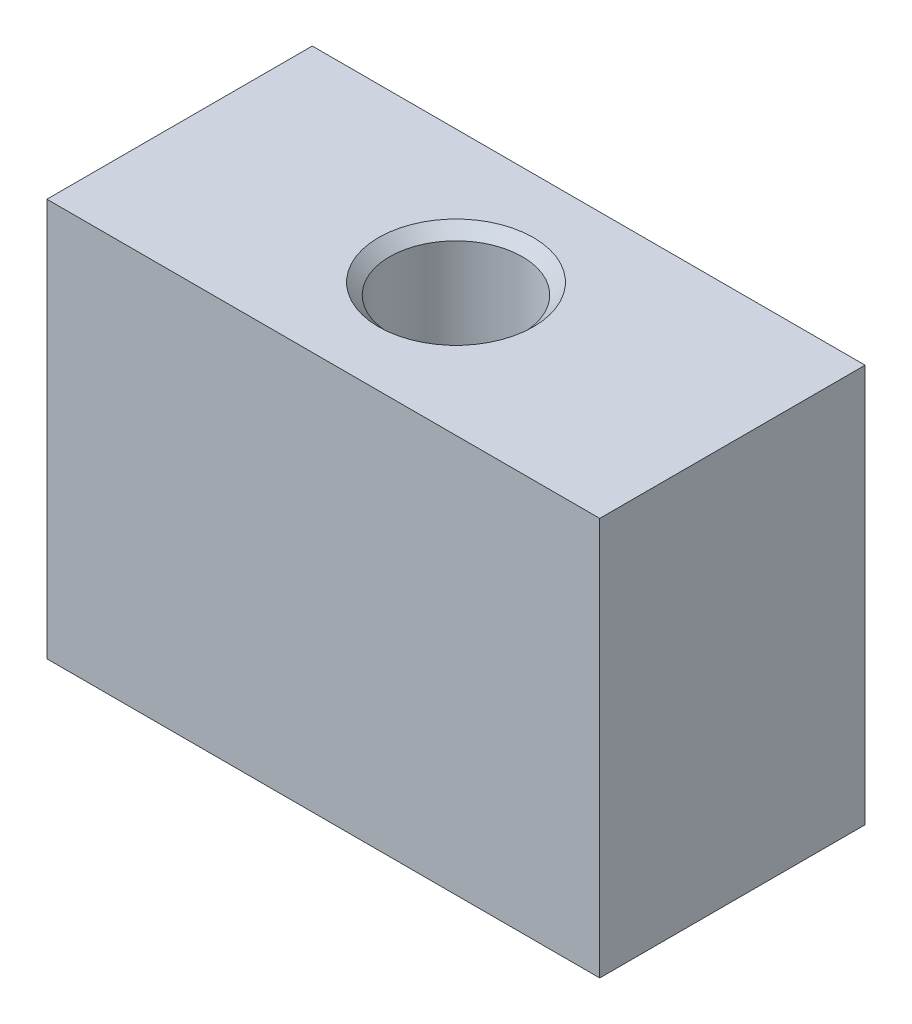
from build123d import *

# Parameters (mm, degrees)
SKETCH1_W           = 25
SKETCH1_H           = 12
BOSS_EXTRUDE1_DEPTH = 18
SKETCH2_R           = 3
CUT_EXTRUDE1_DEPTH  = 23.721135535
CHAMFER1_SIZE       = 0.5


with BuildPart() as part:
    # Sketch1 → Boss-Extrude1 (new body)
    with BuildSketch(Plane(origin=(0, 0, 0), x_dir=(1, 0, 0), z_dir=(0, 1, 0))):
        Rectangle(SKETCH1_W, SKETCH1_H)
    extrude(amount=BOSS_EXTRUDE1_DEPTH)

    # Sketch2 → Cut-Extrude1 (cut, through all)
    with BuildSketch(Plane(origin=(0, 0, 0), x_dir=(1, 0, 0), z_dir=(0, 1, 0))):
        with Locations(Location((0, 0, 0), (0, 0, 270))):
            Circle(SKETCH2_R)
    extrude(amount=CUT_EXTRUDE1_DEPTH, mode=Mode.SUBTRACT)

    # Chamfer1
    chamfer1_edges = [part.edges().sort_by_distance(p)[0] for p in [
        (0, 0, -3),
        (0, 18, -3),
    ]]
    chamfer(chamfer1_edges, length=CHAMFER1_SIZE)


solid = part.part
